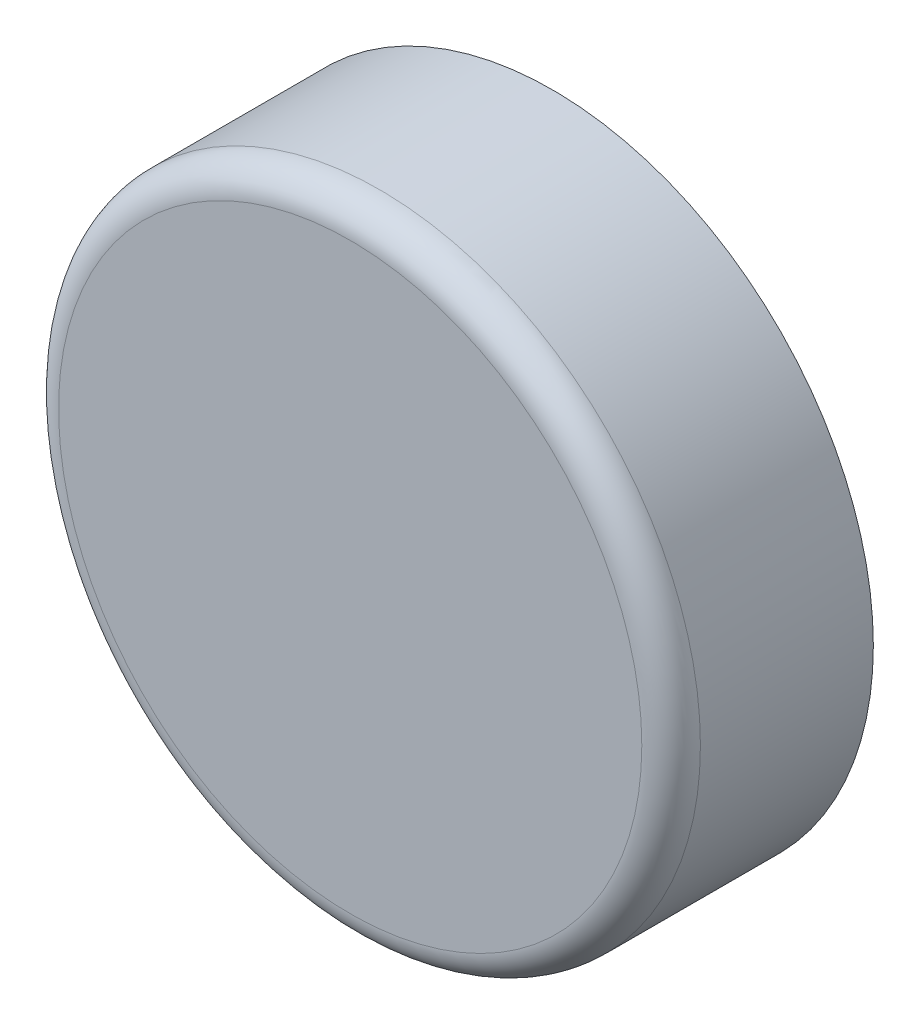
SolidWorks part; units mm, degrees
ref_plane "Front Plane" through (0, 0, 0) normal (0, 0, 1) x (1, 0, 0)
ref_plane "Top Plane" through (0, 0, 0) normal (0, 1, 0) x (1, 0, 0)
ref_plane "Right Plane" through (0, 0, 0) normal (1, 0, 0) x (0, 0, -1)
sketch "Sketch1" plane through (0, 0, 0) normal (0, 0, 1) x (1, 0, 0)
  circle A0 centre (0, 0) radius 109.5
  dimension "D1" = 219
extrude "Boss-Extrude1" add sketch "Sketch1" along normal blind 69 contours A0
shell "Shell1" thickness 6
fillet "Fillet1" radius 10 1 edges at (109.5, 0, 69)
fillet "Fillet2" radius 4 1 edges at (103.5, 0, 63)
